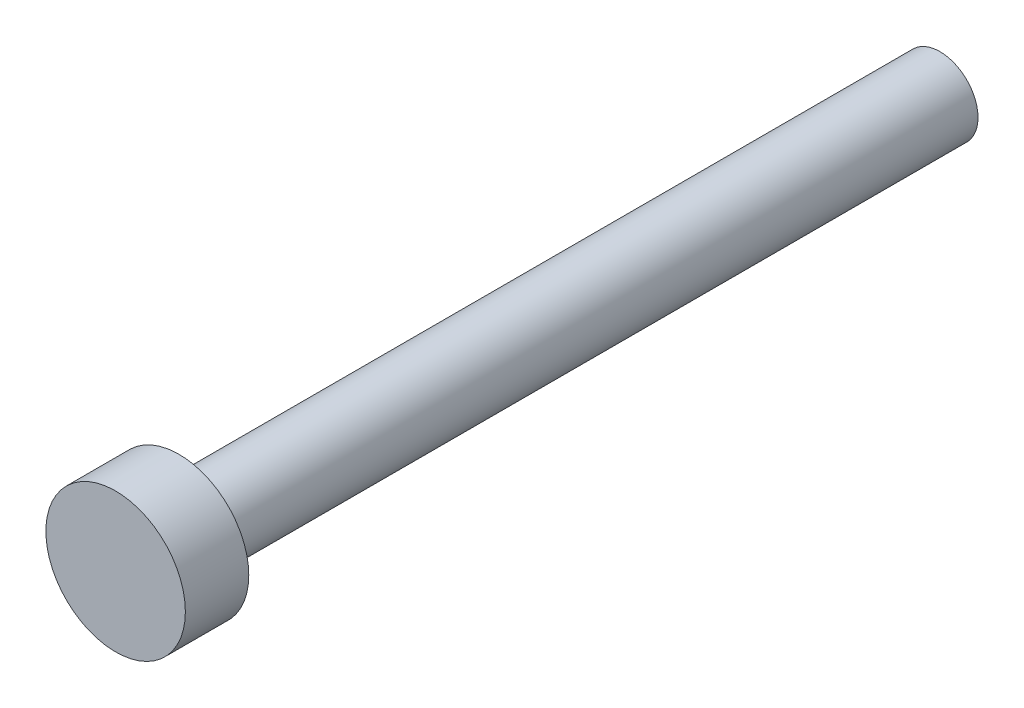
from build123d import *

# Parameters (mm, degrees)
SKETCH_1_R      = 1.5
EXTRUDE_1_DEPTH = 30
SKETCH_2_R      = 2.75
EXTRUDE_2_DEPTH = 2.5


with BuildPart() as part:
    # 草图1 → 凸台-拉伸1 (new body)
    with BuildSketch(Plane.XY):
        Circle(SKETCH_1_R)
    extrude(amount=-EXTRUDE_1_DEPTH)

    # 草图2 → 凸台-拉伸2 (add)
    with BuildSketch(Plane.XY):
        Circle(SKETCH_2_R)
    extrude(amount=EXTRUDE_2_DEPTH)


solid = part.part
